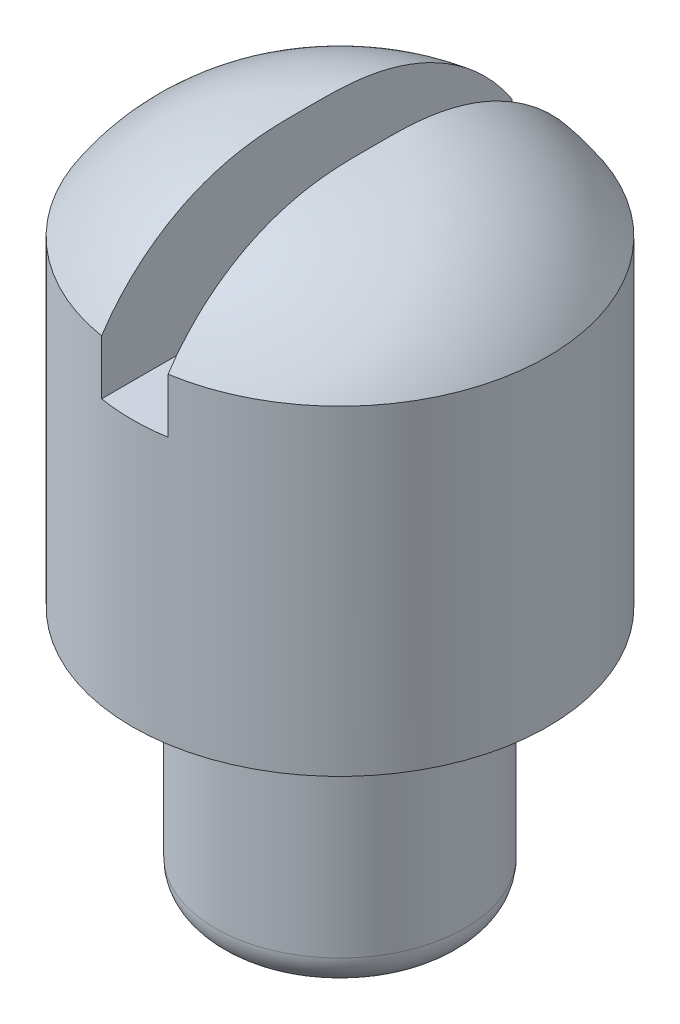
SolidWorks part; units mm, degrees
ref_plane "Front Plane" through (0, 0, 0) normal (0, 0, 1) x (1, 0, 0)
ref_plane "Top Plane" through (0, 0, 0) normal (0, 1, 0) x (1, 0, 0)
ref_plane "Right Plane" through (0, 0, 0) normal (1, 0, 0) x (0, 0, -1)
other "Configuration Table"
sketch "Sketch1" plane through (0, 0, 0) normal (0, 0, 1) x (1, 0, 0)
  line L0 (0, 0) -> (0, 5.0565) construction
  line L1 (0, 0) -> (-1.5, 0)
  line L2 (-1.5, 0) -> (-1.5, 3)
  line L3 (-1.5, 3) -> (-2.5, 3)
  line L4 (-2.5, 3) -> (-2.5, 6.8565)
  line L8 (-0.4, 6.8565) -> (-0.4, 10.2177) construction
  line L9 (-1.7573, 8) -> (1.2914, 8) construction
  line L10 (0, 5.0565) -> (0, 0)
  line L12 (0, 5.0565) -> (0, 8)
  line L13 (0, 8) -> (-0.4, 8)
  arc A2 (-0.4, 8) -> (-2.5, 6.8565) centre (-0.4, 5.5) ccw
  dimension "D1" = 5
  dimension "D2" = 3
  dimension "D3" = 1.5
  dimension "D4" = 2.5
  dimension "D7" = 8
  dimension "D8" = 5
revolve "Revolve1" add sketch "Sketch1" angle 360 about L10
fillet "Fillet1" radius 0.4 1 edges at (0, 3, 1.5)
fillet "Fillet2" radius 0.4 1 edges at (0, 0, 1.5)
sketch "Sketch3" plane through (0, 0, 0) normal (0, 0, 1) x (1, 0, 0)
  line L1 (-0.4, 8) -> (0.4, 8)
  line L2 (-0.4, 8) -> (-0.4, 6.2)
  line L3 (-0.4, 6.2) -> (0.4, 6.2)
  line L4 (0.4, 8) -> (0.4, 6.2)
  dimension "D1" = 0.8
  dimension "D2" = 1.8
extrude "Cut-Extrude1" cut sketch "Sketch3" against normal mid plane 10
